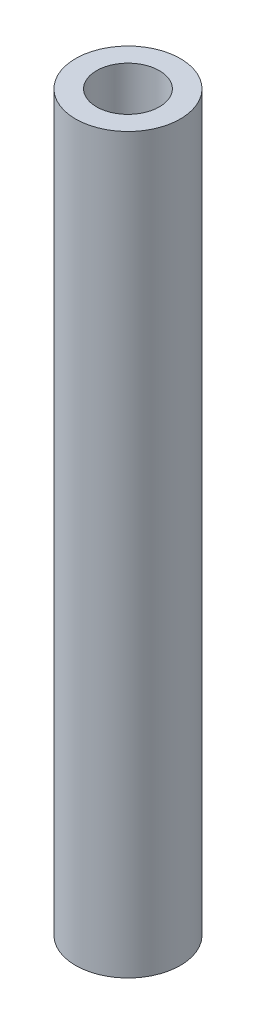
SolidWorks part; units mm, degrees
ref_plane "Front Plane" through (0, 0, 0) normal (0, 0, 1) x (1, 0, 0)
ref_plane "Top Plane" through (0, 0, 0) normal (0, 1, 0) x (1, 0, 0)
ref_plane "Right Plane" through (0, 0, 0) normal (1, 0, 0) x (0, 0, -1)
sketch "Sketch1" plane through (0, 0, 0) normal (0, 1, 0) x (1, 0, 0)
  circle A0 centre (0, 0) radius 2.5
  circle A1 centre (0, 0) radius 1.5
  dimension "D1" = 5
  dimension "D2" = 3
extrude "Boss-Extrude1" add sketch "Sketch1" along normal blind 35
cosmetic thread "Cosmetic Thread1" parameters "D1"=5, "D2"=4
sketch "Sketch2" plane through (0, 0, 0) normal (0, -1, 0) x (1, 0, 0)
  circle A0 centre (0, 0) radius 1.5 construction
  circle A1 centre (0, 0) radius 1.5
  circle A2 centre (0, 0) radius 0.5
  dimension "D1" = 1
extrude "Boss-Extrude2" add sketch "Sketch2" against normal blind 2
